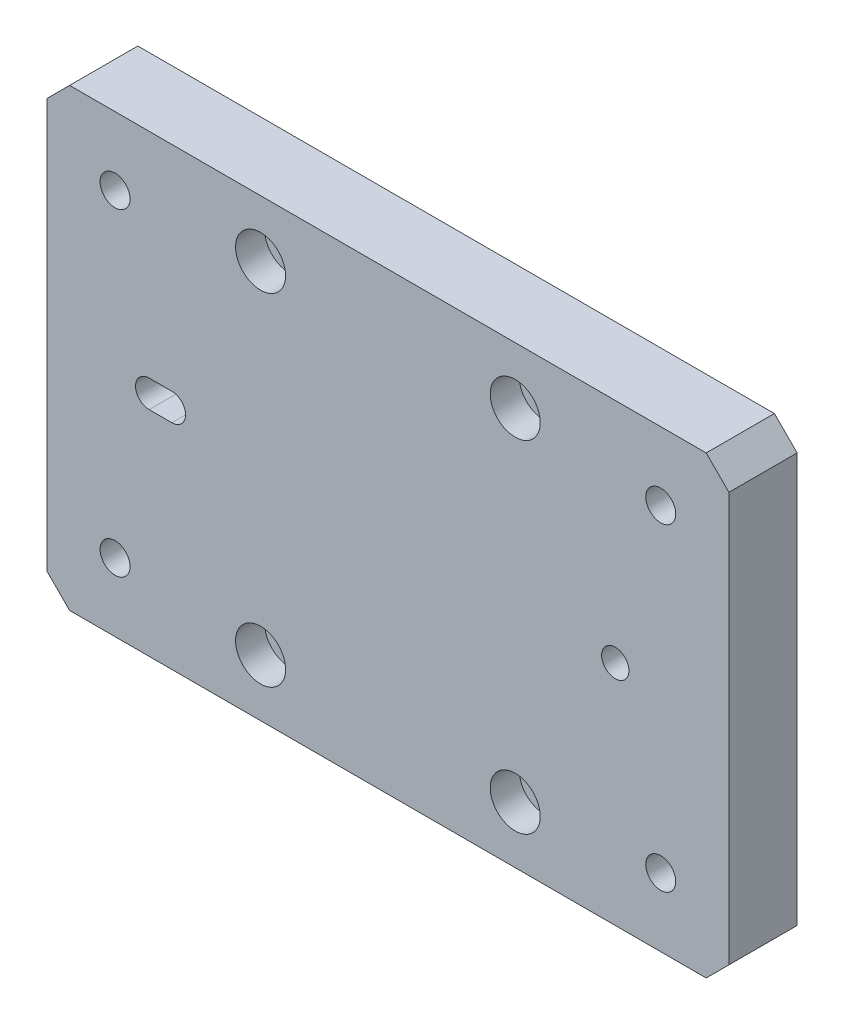
from build123d import *

# Parameters (mm, degrees)
SKETCH_1_W                   = 150
SKETCH_1_H                   = 100
EXTRUDE_1_DEPTH              = 7.5
HOLE_WIZARD_M6_1_D           = 6.6
HOLE_WIZARD_M6_1_CBORE_D     = 11
HOLE_WIZARD_M6_1_CBORE_DEPTH = 6.4
CHAMFER_1_SIZE               = 5
HOLE_WIZARD_M6_2_D           = 6.6
HOLE_WIZARD_M6_2_CBORE_D     = 11
HOLE_WIZARD_M6_2_CBORE_DEPTH = 8
MM_1_D                       = 6
CUT_EXTRUDE_1_DEPTH          = 92.378334412


with BuildPart() as part:
    # 草图1 → 凸台-拉伸1 (new, symmetric)
    with BuildSketch(Plane.XY):
        Rectangle(SKETCH_1_W, SKETCH_1_H)
    extrude(amount=EXTRUDE_1_DEPTH, both=True)

    # M6 六角凹头螺钉的柱形沉头孔1 (through all)
    with Locations(Plane.XY.offset(7.5)):
        with Locations((-28, -37.5), (-28, 37.5), (28, 37.5), (28, -37.5)):
            CounterBoreHole(HOLE_WIZARD_M6_1_D / 2, HOLE_WIZARD_M6_1_CBORE_D / 2, HOLE_WIZARD_M6_1_CBORE_DEPTH)

    # 倒角1
    chamfer_1_edges = [part.edges().sort_by_distance(p)[0] for p in [
        (75, -50, 0),
        (-75, -50, 0),
        (-75, 50, 0),
        (75, 50, 0),
    ]]
    chamfer(chamfer_1_edges, length=CHAMFER_1_SIZE)

    # M6 六角凹头螺钉的柱形沉头孔2 (through all)
    with Locations(Plane(origin=(0, 0, -7.5), x_dir=(-1, 0, 0), z_dir=(0, 0, -1))):
        with Locations((-60, -35), (-60, 35), (60, 35), (60, -35)):
            CounterBoreHole(HOLE_WIZARD_M6_2_D / 2, HOLE_WIZARD_M6_2_CBORE_D / 2, HOLE_WIZARD_M6_2_CBORE_DEPTH)

    # 大小mm 暗销孔1 (through all)
    with Locations(Plane(origin=(0, 0, -7.5), x_dir=(-1, 0, 0), z_dir=(0, 0, -1))):
        with Locations((50, 0), (-50, 0)):
            Hole(MM_1_D / 2)

    # 草图8 → 切除-拉伸1 (cut, through all)
    with BuildSketch(Plane(origin=(0, 0, -7.5), x_dir=(-1, 0, 0), z_dir=(0, 0, -1))):
        with BuildLine():
            Line((47.5, 3), (52.5, 3))
            ThreePointArc((52.5, 3), (55.5, 0), (52.5, -3))
            Line((52.5, -3), (47.5, -3))
            ThreePointArc((47.5, -3), (44.5, 0), (47.5, 3))
        make_face()
    extrude(amount=-CUT_EXTRUDE_1_DEPTH, mode=Mode.SUBTRACT)


solid = part.part
